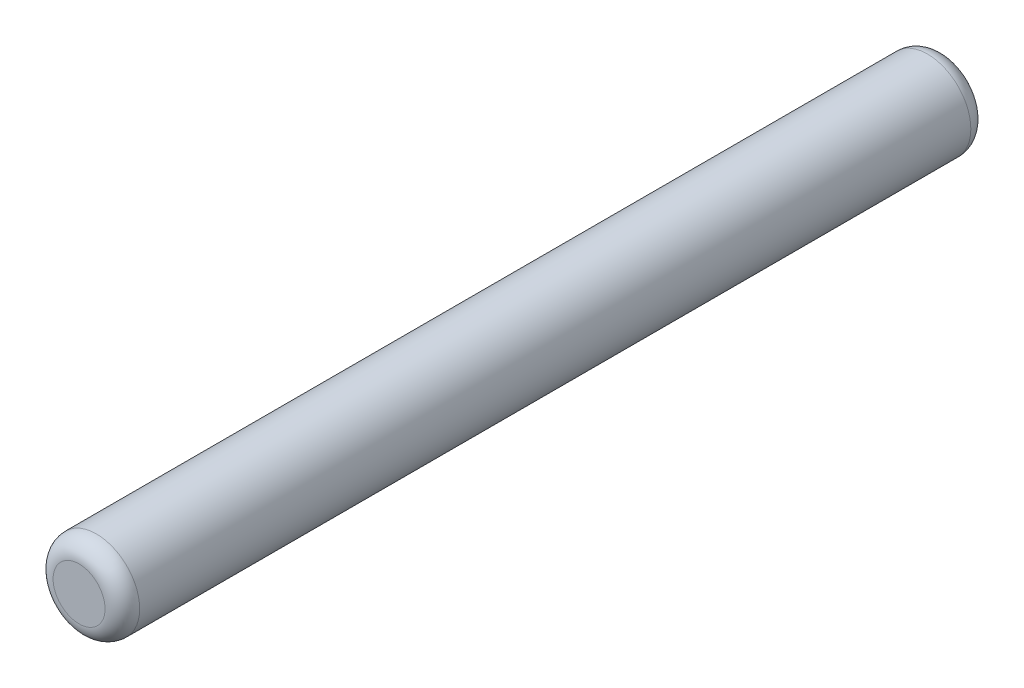
from build123d import *

# Parameters (mm, degrees)
SKETCH1_R           = 0.75
BOSS_EXTRUDE1_DEPTH = 15
FILLET1_R           = 0.3


with BuildPart() as part:
    # Sketch1 → Boss-Extrude1 (new body)
    with BuildSketch(Plane.XY):
        Circle(SKETCH1_R)
    extrude(amount=BOSS_EXTRUDE1_DEPTH)

    # Fillet1
    fillet1_edges = [part.edges().sort_by_distance(p)[0] for p in [
        (-0.75, 0, 0),
        (-0.75, 0, 15),
    ]]
    fillet(fillet1_edges, radius=FILLET1_R)


solid = part.part
